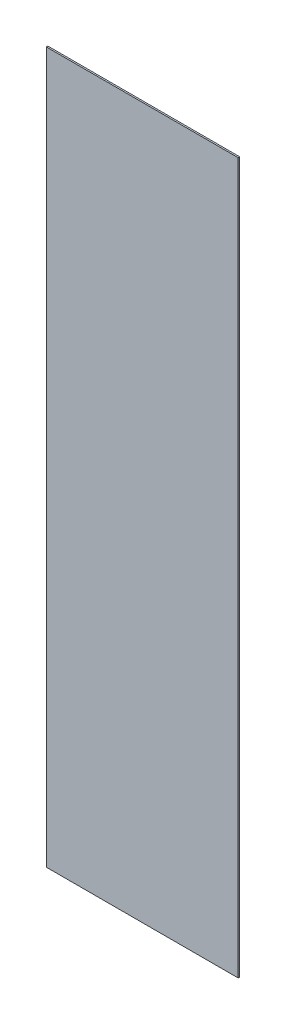
from build123d import *

# Parameters (mm, degrees)
SKETCH_1_W      = 624
SKETCH_1_H      = 2310
EXTRUDE_1_DEPTH = 5


with BuildPart() as part:
    # 草图1 → 凸台-拉伸1 (new body)
    with BuildSketch(Plane.XY):
        Rectangle(SKETCH_1_W, SKETCH_1_H)
    extrude(amount=EXTRUDE_1_DEPTH)


solid = part.part
